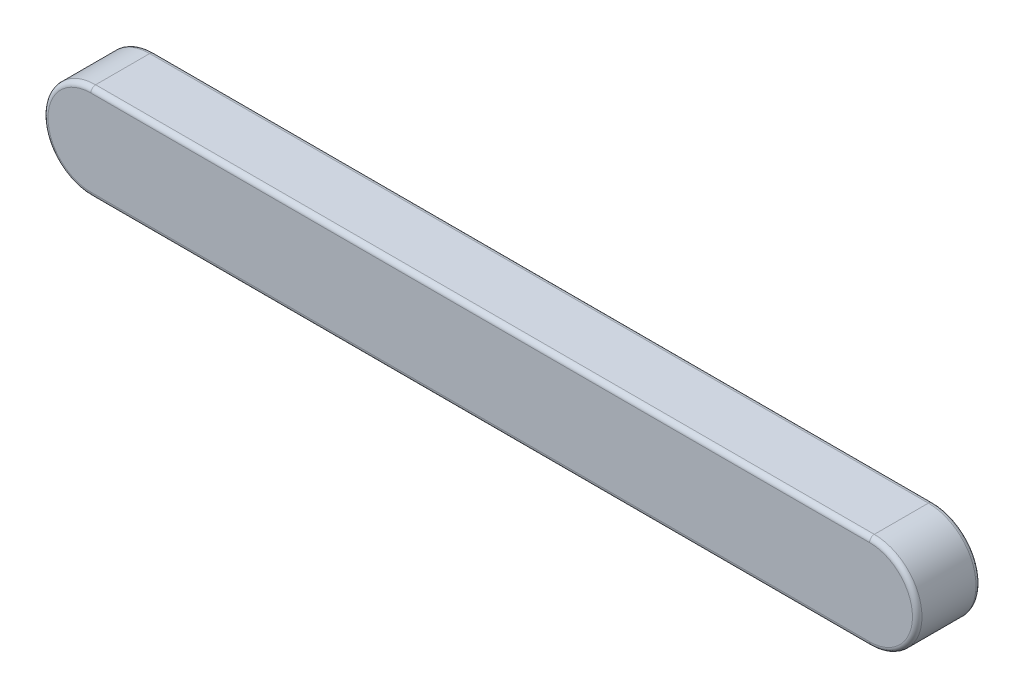
SolidWorks part; units mm, degrees
material "45"
ref_plane "基准面1" through (0, 0, 0) normal (0, 0, 1) x (1, 0, 0)
ref_plane "基准面2" through (0, 0, 0) normal (0, 1, 0) x (1, 0, 0)
ref_plane "基准面3" through (0, 0, 0) normal (1, 0, 0) x (0, 0, -1)
sketch "尺寸草图" plane through (0, 0, 0) normal (0, 0, 1) x (1, 0, 0)
  line L0 (-55, 0) -> (55, 0) construction
  point P3 (-8, 0)
  point P4 (-0.6, 0)
  point P5 (0, 0)
  point P8 (-12, 0)
  point P11 (0, 0)
sketch "草图1" plane through (0, 0, 0) normal (0, 0, 1) x (1, 0, 0)
  line L0 (-28.0599, 0) -> (30.562, 0) construction
  line L1 (-49, 6) -> (49, 6)
  line L2 (-49, -6) -> (49, -6)
  line L3 (0, 2.9108) -> (0, -2.1805) construction
  arc A0 (-49, 6) -> (-49, -6) centre (-49, 0) ccw
  arc A1 (49, 6) -> (49, -6) centre (49, 0) cw
extrude "基体-拉伸" add sketch "草图1" along normal blind 8
fillet "圆角1" radius 0.6 8 edges at (55, 0, 8) (0, 6, 8) (-55, 0, 8) (0, 6, 0) (55, 0, 0) (0, -6, 0) (-55, 0, 0) (0, -6, 8)
equation "\"D3@草图1\" = \"L@尺寸草图\""
equation "\"D1@草图1\" = \"b@尺寸草图\" / 2"
equation "\"D1@圆角1\" = \"r@尺寸草图\""
equation "\"D1@基体-拉伸\" = \"h@尺寸草图\""
